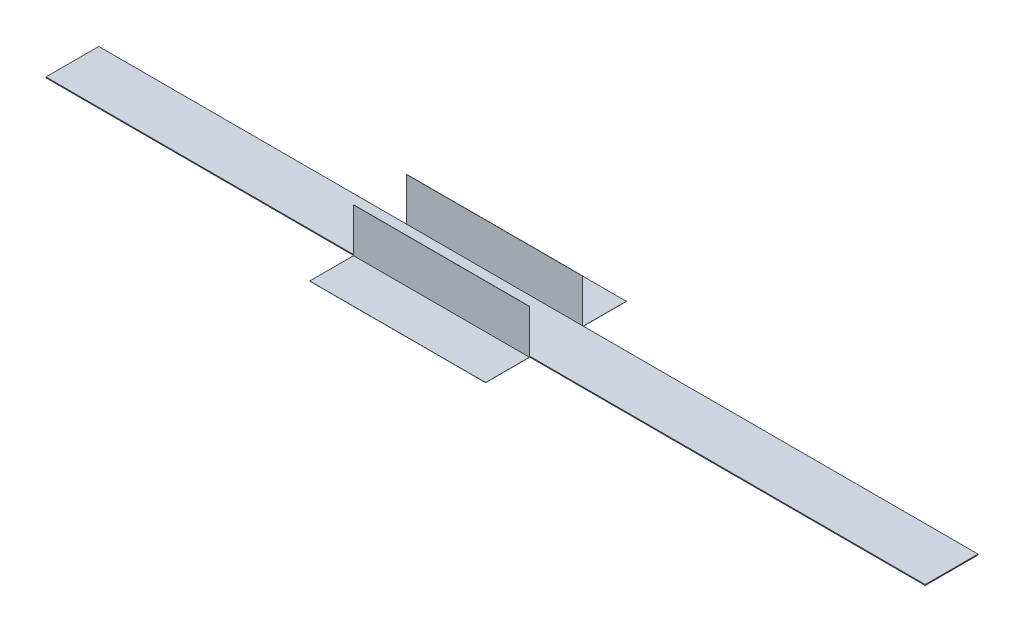
SolidWorks part; units mm, degrees
ref_plane "Front Plane" through (0, 0, 0) normal (0, 0, 1) x (1, 0, 0)
ref_plane "Top Plane" through (0, 0, 0) normal (0, 1, 0) x (1, 0, 0)
ref_plane "Right Plane" through (0, 0, 0) normal (1, 0, 0) x (0, 0, -1)
sketch "Sketch1" plane through (0, 0, 0) normal (0, 0, 1) x (1, 0, 0)
  line L0 (0, 0) -> (100, 0)
  dimension "D1" = 100
extrude "Extrude-Thin1" add sketch "Sketch1" along normal mid plane 6 thin thin type mid plane wall 0.1
sketch "Sketch2" plane through (0, -0.05, 0) normal (0, -1, 0) x (1, 0, 0)
  line L0 (0, 0) -> (63.5697, 0) construction
  line L1 (35, -8) -> (55, -8)
  line L2 (35, -8) -> (35, 8)
  line L3 (35, 8) -> (55, 8)
  line L4 (55, -8) -> (55, 8)
  line L5 (35, -8) -> (55, 8) construction
  line L6 (35, 8) -> (55, -8) construction
  line L8 (0, 3) -> (0, -3) construction
  point P0 (45, 0)
  dimension "D1" = 20
  dimension "D2" = 16
  dimension "D3" = 45
extrude "Boss-Extrude1" add sketch "Sketch2" along normal blind 0.02
sketch "Sketch3" plane through (0, -0.05, 0) normal (0, 1, 0) x (1, 0, 0)
  line L0 (55, 8) -> (55, 3) construction
  line L1 (35, 3) -> (55, 3)
  line L2 (35, 3) -> (35, 3.02)
  line L3 (35, 3.02) -> (55, 3.02)
  line L4 (55, 3) -> (55, 3.02)
  line L6 (0, 0) -> (67.9455, 0) construction
  line L7 (55, -3) -> (55, -3.02)
  line L8 (35, -3.02) -> (55, -3.02)
  line L9 (35, -3) -> (35, -3.02)
  line L10 (35, -3) -> (55, -3)
  dimension "D1" = 0.02
extrude "Boss-Extrude2" add sketch "Sketch3" along normal blind 5
